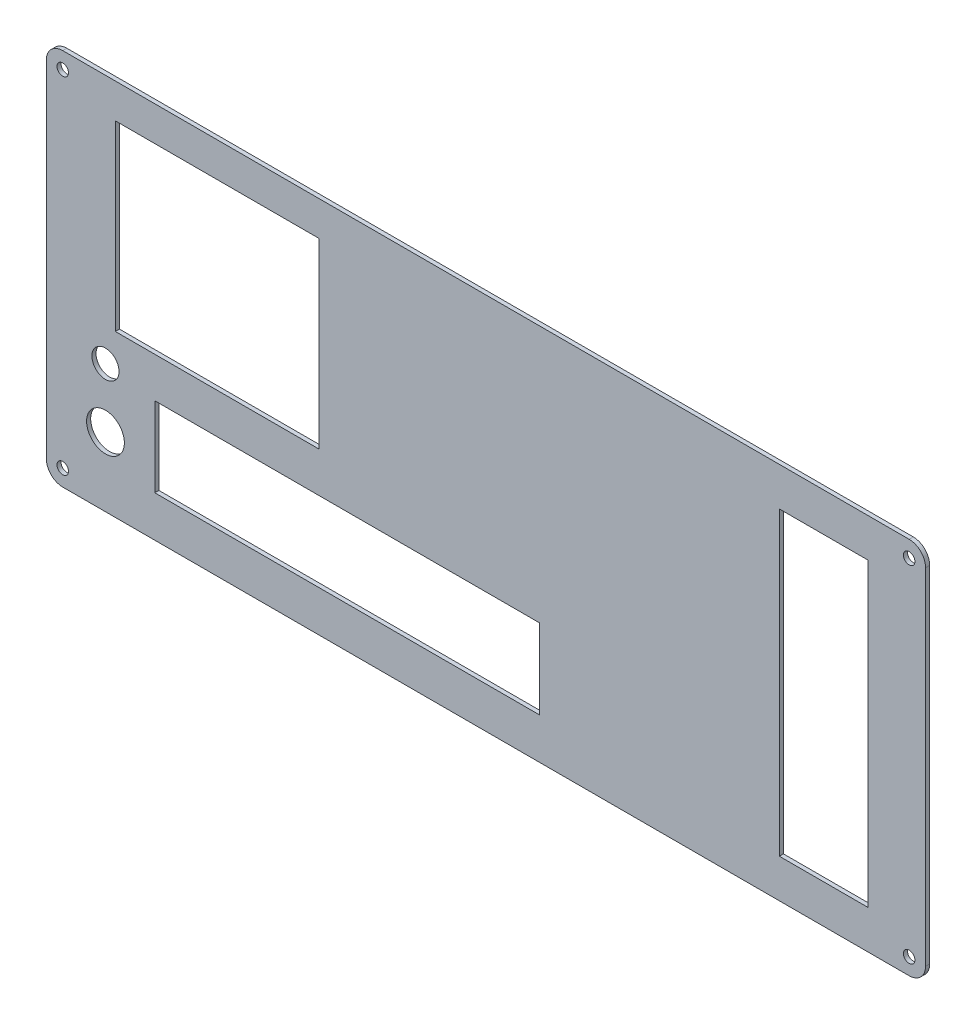
SolidWorks part; units mm, degrees
material "Plain Carbon Steel"
ref_plane "Front Plane" through (0, 0, 0) normal (0, 0, 1) x (1, 0, 0)
ref_plane "Top Plane" through (0, 0, 0) normal (0, 1, 0) x (1, 0, 0)
ref_plane "Right Plane" through (0, 0, 0) normal (1, 0, 0) x (0, 0, -1)
sketch "Sketch1" plane through (0, 0, 0) normal (0, 0, 1) x (1, 0, 0)
  line L1 (0, 0) -> (535, 0)
  line L2 (0, 0) -> (0, -230)
  line L3 (0, -230) -> (535, -230)
  line L4 (535, 0) -> (535, -230)
  dimension "D1" = 535
  dimension "D2" = 230
extrude "Boss-Extrude1" add sketch "Sketch1" along normal blind 2.5
fillet "Fillet1" radius 10 4 edges at (0, -230, 1.25) (535, -230, 1.25) (535, 0, 1.25) (0, 0, 1.25)
sketch "Sketch2" plane through (0, 0, 2.5) normal (0, 0, 1) x (1, 0, 0)
  line L0 (525, 0) -> (10, 0) construction
  line L1 (0, -10) -> (0, -220) construction
  circle A0 centre (10, -10) radius 3.5
  dimension "D3" = 7
  dimension "D1" = 10
  dimension "D2" = 10
extrude "Cut-Extrude1" cut sketch "Sketch2" against normal blind 2.5
pattern_linear "LPattern1" count 2 spacing 515 along (1, 0, 0) count 2 spacing 210 along (0, -1, 0) of "Cut-Extrude1"
sketch "Sketch3" plane through (0, 0, 2.5) normal (0, 0, 1) x (1, 0, 0)
  line L0 (525, 0) -> (10, 0) construction
  line L1 (42, -21) -> (166, -21)
  line L2 (42, -21) -> (42, -132)
  line L3 (42, -132) -> (166, -132)
  line L4 (166, -21) -> (166, -132)
  line L5 (0, -10) -> (0, -220) construction
  dimension "D1" = 124
  dimension "D2" = 111
  dimension "D3" = 21
  dimension "D4" = 42
extrude "Cut-Extrude2" cut sketch "Sketch3" against normal blind 2.5
sketch "Sketch4" plane through (0, 0, 2.5) normal (0, 0, 1) x (1, 0, 0)
  line L0 (0, -10) -> (0, -220) construction
  line L1 (66, -156.5) -> (300, -156.5)
  line L2 (66, -156.5) -> (66, -205)
  line L3 (66, -205) -> (300, -205)
  line L4 (300, -156.5) -> (300, -205)
  line L5 (10, -230) -> (525, -230) construction
  dimension "D1" = 234
  dimension "D2" = 48.5
  dimension "D3" = 66
  dimension "D4" = 25
extrude "Cut-Extrude3" cut sketch "Sketch4" against normal blind 2.5
sketch "Sketch5" plane through (0, 0, 2.5) normal (0, 0, 1) x (1, 0, 0)
  line L0 (0, -10) -> (0, -220) construction
  line L1 (10, -230) -> (525, -230) construction
  circle A0 centre (36, -188) radius 11.5
  dimension "D3" = 23
  dimension "D1" = 36
  dimension "D2" = 42
extrude "Cut-Extrude4" cut sketch "Sketch5" against normal blind 2.5
sketch "Sketch7" plane through (0, 0, 2.5) normal (0, 0, 1) x (1, 0, 0)
  line L0 (0, -10) -> (0, -220) construction
  line L1 (10, -230) -> (525, -230) construction
  circle A0 centre (36, -152) radius 8.25
  dimension "D3" = 16.5
  dimension "D1" = 36
  dimension "D2" = 78
extrude "Cut-Extrude5" cut sketch "Sketch7" against normal blind 2.5
sketch "Sketch8" plane through (0, 0, 2.5) normal (0, 0, 1) x (1, 0, 0)
  line L0 (535, -220) -> (535, -10) construction
  line L1 (446, -23.5) -> (500, -23.5)
  line L2 (446, -23.5) -> (446, -206.5)
  line L3 (446, -206.5) -> (500, -206.5)
  line L4 (500, -23.5) -> (500, -206.5)
  line L5 (10, -230) -> (525, -230) construction
  dimension "D1" = 183
  dimension "D2" = 54
  dimension "D3" = 35
  dimension "D4" = 23.5
extrude "Cut-Extrude6" cut sketch "Sketch8" against normal blind 2.5
